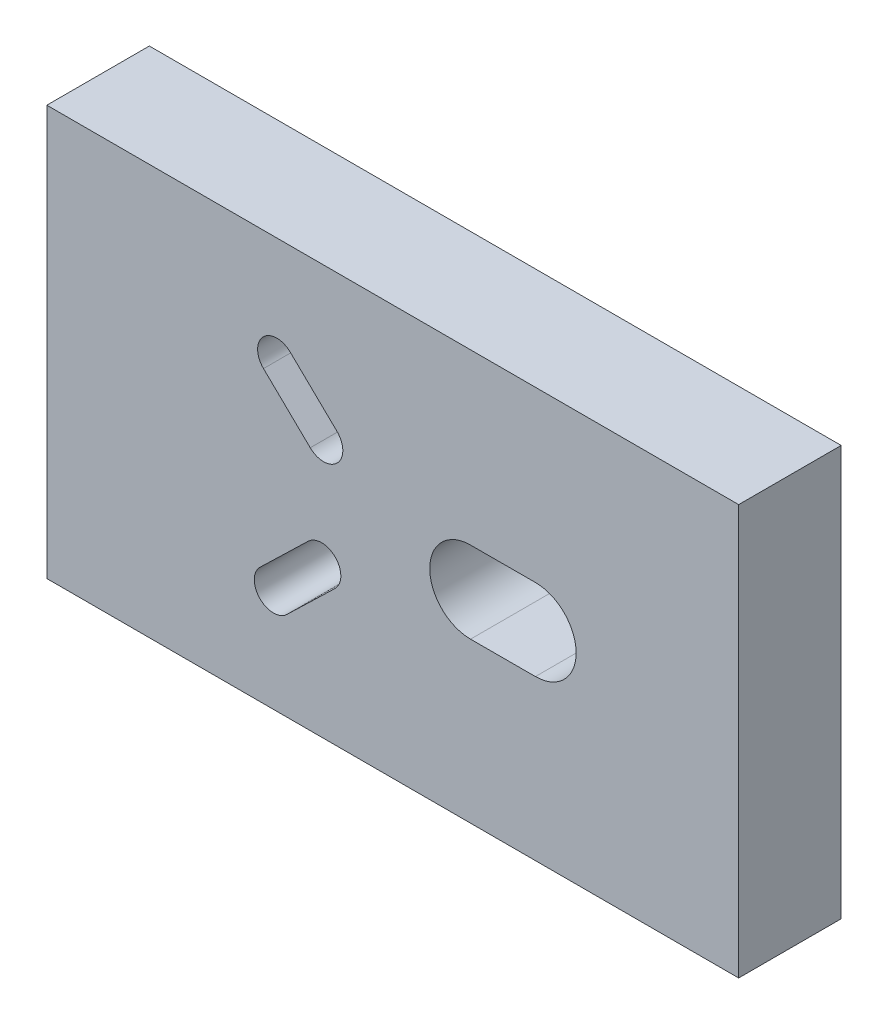
SolidWorks part; units mm, degrees
ref_plane "前视基准面" through (0, 0, 0) normal (0, 0, 1) x (1, 0, 0)
ref_plane "上视基准面" through (0, 0, 0) normal (0, 1, 0) x (1, 0, 0)
ref_plane "右视基准面" through (0, 0, 0) normal (1, 0, 0) x (0, 0, -1)
sketch "草图1" plane through (0, 0, 0) normal (0, 0, 1) x (1, 0, 0)
  line L1 (-9.6011, 4.1182) -> (17.3989, 4.1182)
  line L2 (-9.6011, 4.1182) -> (-9.6011, -11.8818)
  line L3 (-9.6011, -11.8818) -> (17.3989, -11.8818)
  line L4 (17.3989, 4.1182) -> (17.3989, -11.8818)
  dimension "D1" = 27
  dimension "D2" = 16
extrude "凸台-拉伸1" add sketch "草图1" along normal blind 4
sketch "草图2" plane through (0, 0, 4) normal (0, 0, 1) x (1, 0, 0)
  circle A0 centre (1.1999, -1.7816) radius 0.75
  circle A1 centre (1.1225, -6.0568) radius 0.75
  circle A2 centre (9.4654, -4.0695) radius 1.59
extrude "切除-拉伸2" cut sketch "草图2" against normal up to surface (4 mm away) up to face at (3.8989, -3.8818, 0)
sketch "草图3" plane through (0, 0, 4) normal (0, 0, 1) x (1, 0, 0)
  line L0 (6.9319, -2.4815) -> (9.4642, -2.4795)
  line L1 (6.9343, -5.6615) -> (9.4666, -5.6595)
  line L2 (-1.2764, -7.3328) -> (0.6012, -5.5176)
  line L3 (1.6438, -6.596) -> (-0.2339, -8.4112)
  line L4 (-1.146, -0.5569) -> (0.6786, -2.3208)
  line L5 (1.7212, -1.2424) -> (-0.1034, 0.5215)
  arc A0 (6.9319, -2.4815) -> (6.9343, -5.6615) centre (6.9331, -4.0715) ccw
  arc A1 (1.7212, -1.2424) -> (0.6786, -2.3208) centre (1.1999, -1.7816) ccw
  arc A2 (0.6012, -5.5176) -> (1.6438, -6.596) centre (1.1225, -6.0568) ccw
  arc A3 (-0.1034, 0.5215) -> (-1.146, -0.5569) centre (-0.6247, -0.0177) ccw
  arc A4 (-1.2764, -7.3328) -> (-0.2339, -8.4112) centre (-0.7552, -7.872) ccw
  arc A5 (9.4642, -2.4795) -> (9.4666, -5.6595) centre (9.4654, -4.0695) ccw
extrude "切除-拉伸3" cut sketch "草图3" against normal up to surface (4 mm away) up to face at (11.0554, -4.0695, 0)
